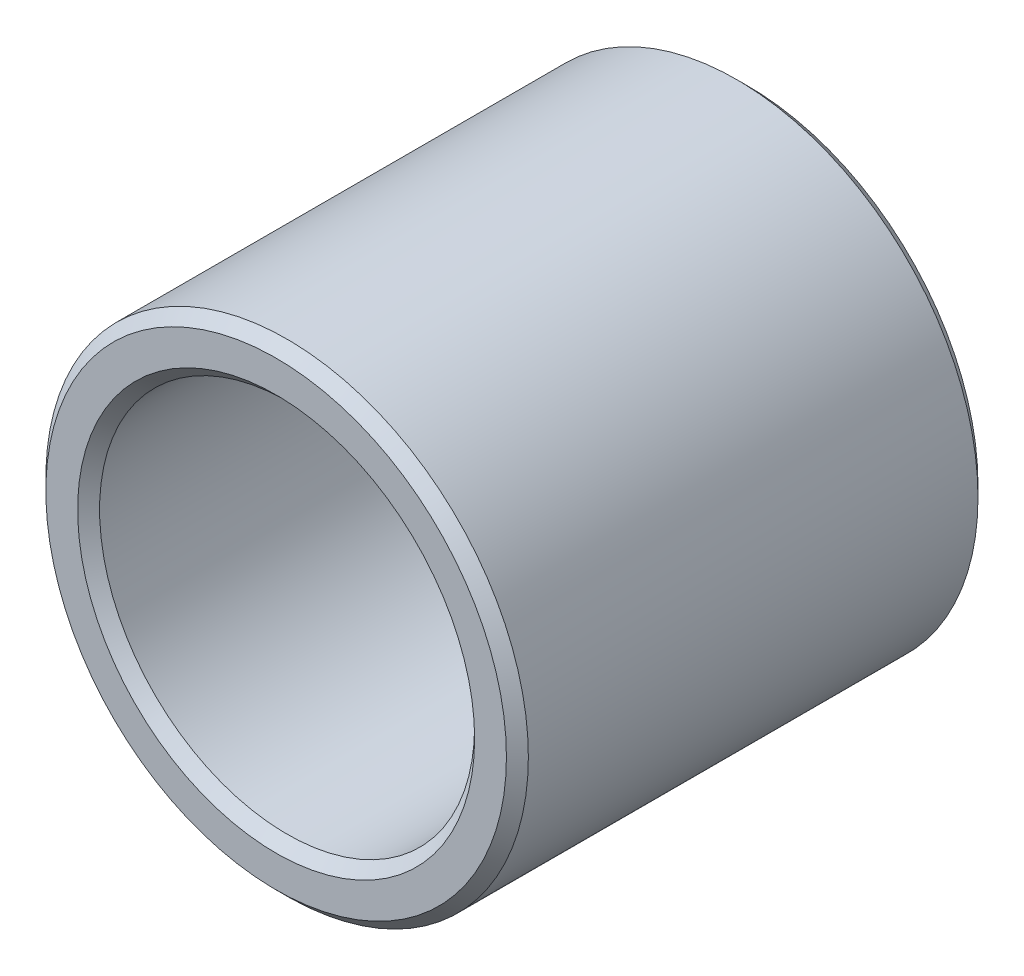
SolidWorks part; units mm, degrees
ref_plane "前视" through (0, 0, 0) normal (0, 0, 1) x (1, 0, 0)
ref_plane "上视" through (0, 0, 0) normal (0, 1, 0) x (1, 0, 0)
ref_plane "右视" through (0, 0, 0) normal (1, 0, 0) x (0, 0, -1)
sketch "草图1" plane through (0, 0, 0) normal (0, 0, 1) x (1, 0, 0)
  circle A0 centre (0, 0) radius 8.55
  circle A1 centre (0, 0) radius 11
  dimension "D1" = 17.1
  dimension "D2" = 22
extrude "凸台-拉伸1" add sketch "草图1" along normal blind 21.5
chamfer "倒角1" distance 0.5 angle 45 4 edges at (8.55, 0, 0) (11, 0, 0) (8.55, 0, 21.5) (11, 0, 21.5)
